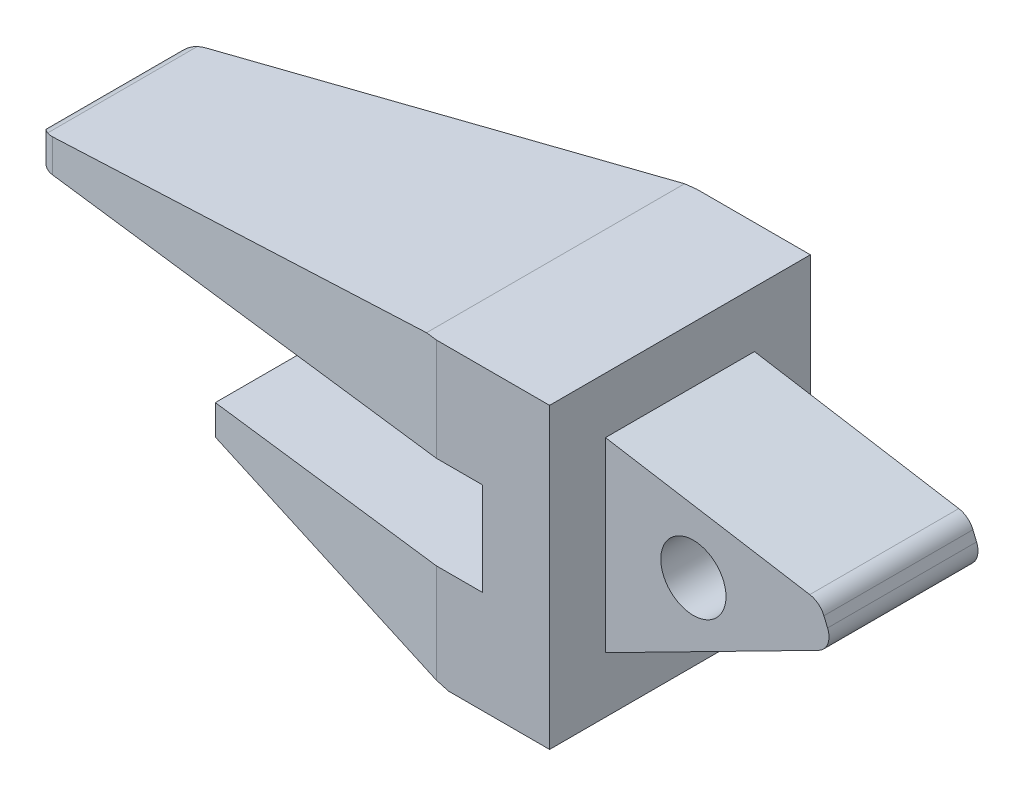
SolidWorks part; units mm, degrees
ref_plane "Front Plane" through (0, 0, 0) normal (0, 0, 1) x (1, 0, 0)
ref_plane "Top Plane" through (0, 0, 0) normal (0, 1, 0) x (1, 0, 0)
ref_plane "Right Plane" through (0, 0, 0) normal (1, 0, 0) x (0, 0, -1)
sketch "Sketch1" plane through (0, 0, 0) normal (0, 1, 0) x (1, 0, 0)
  line L0 (0, 14.6894) -> (0, -14.6894)
  line L1 (153, 35) -> (153, -35)
  line L2 (153, 35) -> (122.6, 35)
  line L3 (122.6, 35) -> (5.2713, 20.6449)
  line L4 (5.2713, -20.6449) -> (122.6, -35)
  line L5 (122.6, -35) -> (153, -35)
  arc A0 (0, -14.6894) -> (5.2713, -20.6449) centre (6, -14.6894) ccw
  arc A1 (0, 14.6894) -> (5.2713, 20.6449) centre (6, 14.6894) cw
  point P9 (0, -20)
  point P12 (0, 20)
  dimension "D8" = 6
  dimension "D1" = 153
  dimension "D2" = 40
  dimension "D3" = 20
  dimension "D4" = 35
  dimension "D5" = 70
  dimension "D6" = 30.4
  dimension "D7" = 30.4
extrude "Boss-Extrude1" add sketch "Sketch1" along normal blind 80
sketch "Sketch2" plane through (0, 0, 0) normal (0, 0, 1) x (1, 0, 0)
  line L0 (153, 80) -> (153, 0) construction
  line L1 (153, 80) -> (153, 0)
  line L4 (5.2713, 80) -> (0, 80) construction
  line L6 (0, 0) -> (5.2713, 0) construction
  line L13 (0, 0) -> (5.2713, 0)
  line L16 (55, 27.5) -> (55, 19.5)
  line L17 (153, 0) -> (125.9, 0)
  line L18 (55, 19.5) -> (125.9, 0)
  line L19 (55, 27.5) -> (135, 27.5)
  line L20 (135, 52.5) -> (135, 27.5)
  line L21 (135, 52.5) -> (0, 52.5)
  line L22 (153, 80) -> (119.6, 80)
  line L23 (0, 52.5) -> (0, 57.0994)
  line L24 (3.3563, 61.0472) -> (119.6, 80)
  arc A0 (0, 57.0994) -> (3.3563, 61.0472) centre (4, 57.0994) cw
  point P19 (0, 60.5)
  dimension "D9" = 4
  dimension "D1" = 98
  dimension "D2" = 19.5
  dimension "D3" = 27.5
  dimension "D4" = 27.1
  dimension "D5" = 18
  dimension "D6" = 25
  dimension "D7" = 33.4
  dimension "D8" = 8
extrude "Cut-Extrude1" cut sketch "Sketch2" against normal through all and the other way through all flip side to cut contours L20 L19 L16 L18 L17 L1 L22 L24 A0 L23 L21
sketch "Sketch3" plane through (0, 0, 0) normal (0, 0, 1) x (1, 0, 0)
  line L0 (153, 80) -> (153, 0) construction
  line L1 (153, 65) -> (153, 15)
  line L2 (153, 15) -> (210.27, 44.1805)
  line L3 (212.6166, 50.5556) -> (211.6379, 52.9089)
  line L4 (207.8379, 55.9216) -> (153, 65)
  arc A0 (210.27, 44.1805) -> (212.6166, 50.5556) centre (208, 48.6355) ccw
  arc A1 (207.8379, 55.9216) -> (211.6379, 52.9089) centre (207.0212, 50.9888) cw
  dimension "D5" = 5
  dimension "D1" = 15
  dimension "D2" = 15
  dimension "D3" = 80.6
  dimension "D4" = 63
  dimension "D6" = 55
extrude "Boss-Extrude2" add sketch "Sketch3" along normal blind 20 and the other way blind 20
hole_wizard "M20 Tapped Hole1" positions "Sketch5" profile "Sketch4" tap size "M20" standard "GB" end condition through all
sketch "Sketch5" plane through (0, 0, 20) normal (0, 0, 1) x (1, 0, 0)
  line L0 (153, 80) -> (153, 0) construction
  line L1 (122.6, 80) -> (153, 80) construction
  point P0 (176.6, 44.2)
  dimension "D1" = 23.6
  dimension "D2" = 35.8
sketch "Sketch4" plane through (176.6, 44.2, 20) normal (1, 0, 0) x (0, -1, 0)
  line L0 (0, 0) -> (0, 55)
  line L1 (0, 55) -> (8.75, 55)
  line L2 (8.75, 55) -> (8.75, 0)
  line L5 (8.75, 0) -> (0, 0)
  line L11 (0, -6.35) -> (0, 107.95) construction
  dimension "通孔螺纹孔钻头直径" = 17.5
  dimension "通孔螺纹孔钻头深度" = 55
cosmetic thread "Cosmetic Thread1" parameters "D2"=20
